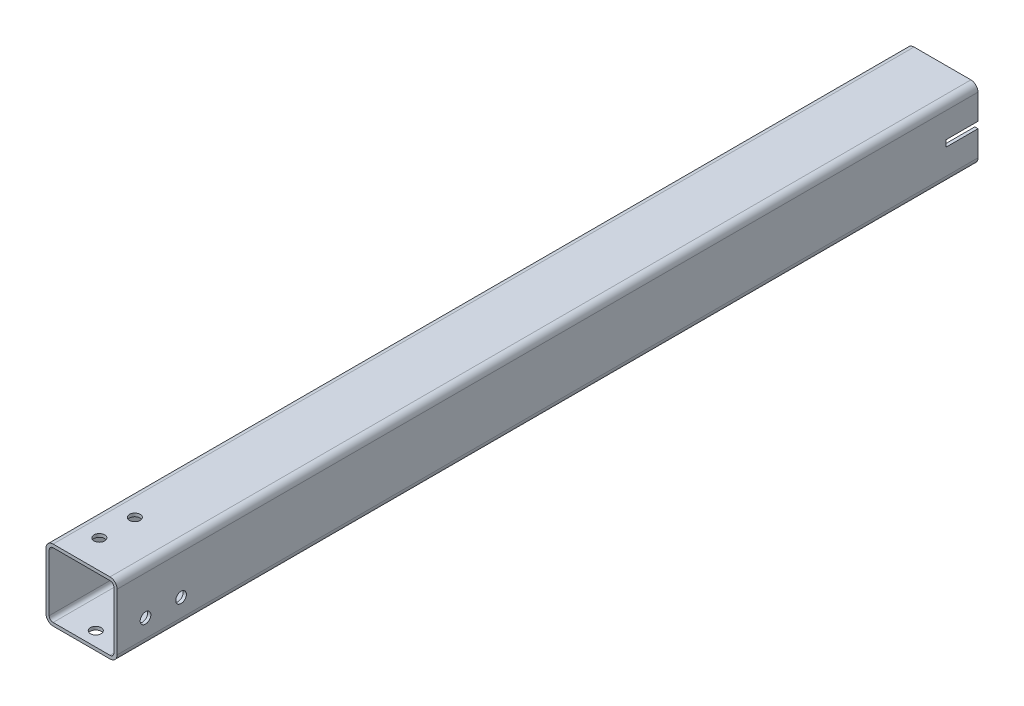
from build123d import *

# Parameters (mm, degrees)
BOSS_EXTRUDE1_DEPTH = 1211
CUT_EXTRUDE1_REACH  = 1218.15
SKETCH_1_R          = 7.5
CUT_EXTRUDE2_REACH  = 1218.15
SKETCH2_R           = 7.5
CUT_EXTRUDE3_REACH  = 1218.15
SKETCH3_R           = 7.5
SKETCH4_W           = 45
SKETCH4_H           = 9
CUT_EXTRUDE4_DEPTH  = 1217.150072976


with BuildPart() as part:
    # Sketch1 → Boss-Extrude1 (new body)
    with BuildSketch(Plane.XY):
        with BuildLine():
            Line((-40, -50), (40, -50))
            ThreePointArc((40, -50), (47.071067812, -47.071067812), (50, -40))
            Line((50, -40), (50, 40))
            ThreePointArc((50, 40), (47.071067812, 47.071067812), (40, 50))
            Line((40, 50), (-40, 50))
            ThreePointArc((-40, 50), (-47.071067812, 47.071067812), (-50, 40))
            Line((-50, 40), (-50, -40))
            ThreePointArc((-50, -40), (-47.071067812, -47.071067812), (-40, -50))
        make_face()
        with BuildLine():
            Line((-40, -45.5), (40, -45.5))
            ThreePointArc((40, -45.5), (43.889087297, -43.889087297), (45.5, -40))
            Line((45.5, -40), (45.5, 40))
            ThreePointArc((45.5, 40), (43.889087297, 43.889087297), (40, 45.5))
            Line((40, 45.5), (-40, 45.5))
            ThreePointArc((-40, 45.5), (-43.889087297, 43.889087297), (-45.5, 40))
            Line((-45.5, 40), (-45.5, -40))
            ThreePointArc((-45.5, -40), (-43.889087297, -43.889087297), (-40, -45.5))
        make_face(mode=Mode.SUBTRACT)
    extrude(amount=BOSS_EXTRUDE1_DEPTH)

    # 草图1 → Cut-Extrude1 (cut, up to next)
    with BuildSketch(Plane(origin=(50, 0, 0), x_dir=(0, 0, -1), z_dir=(1, 0, 0)), mode=Mode.PRIVATE) as cut_extrude1_sk1:
        with Locations((-1171, -15)):
            Circle(SKETCH_1_R)
    cut_extrude1_tool1 = extrude(cut_extrude1_sk1.sketch, amount=-CUT_EXTRUDE1_REACH, mode=Mode.PRIVATE) & part.part
    # 草图1 → Cut-Extrude1 (cut, up to next)
    with BuildSketch(Plane(origin=(50, 0, 0), x_dir=(0, 0, -1), z_dir=(1, 0, 0)), mode=Mode.PRIVATE) as cut_extrude1_sk2:
        with Locations((-1121, -15)):
            Circle(SKETCH_1_R)
    cut_extrude1_tool2 = extrude(cut_extrude1_sk2.sketch, amount=-CUT_EXTRUDE1_REACH, mode=Mode.PRIVATE) & part.part
    add(cut_extrude1_tool1.solids().sort_by_distance((50, -15, 1171))[0], mode=Mode.SUBTRACT)
    add(cut_extrude1_tool2.solids().sort_by_distance((50, -15, 1121))[0], mode=Mode.SUBTRACT)

    # Sketch2 → Cut-Extrude2 (cut, up to next)
    with BuildSketch(Plane.XZ.offset(50), mode=Mode.PRIVATE) as cut_extrude2_sk1:
        with Locations(Location((0, 1191, 0), (0, 0, 270))):
            Circle(SKETCH2_R)
    cut_extrude2_tool1 = extrude(cut_extrude2_sk1.sketch, amount=-CUT_EXTRUDE2_REACH, mode=Mode.PRIVATE) & part.part
    # Sketch2 → Cut-Extrude2 (cut, up to next)
    with BuildSketch(Plane.XZ.offset(50), mode=Mode.PRIVATE) as cut_extrude2_sk2:
        with Locations(Location((0, 1121, 0), (0, 0, 270))):
            Circle(SKETCH2_R)
    cut_extrude2_tool2 = extrude(cut_extrude2_sk2.sketch, amount=-CUT_EXTRUDE2_REACH, mode=Mode.PRIVATE) & part.part
    # Sketch2 → Cut-Extrude2 (cut, up to next)
    with BuildSketch(Plane.XZ.offset(50), mode=Mode.PRIVATE) as cut_extrude2_sk3:
        with Locations(Location((0, 20, 0), (0, 0, 270))):
            Circle(SKETCH2_R)
    cut_extrude2_tool3 = extrude(cut_extrude2_sk3.sketch, amount=-CUT_EXTRUDE2_REACH, mode=Mode.PRIVATE) & part.part
    add(cut_extrude2_tool1.solids().sort_by_distance((0, -50, 1191))[0], mode=Mode.SUBTRACT)
    add(cut_extrude2_tool2.solids().sort_by_distance((0, -50, 1121))[0], mode=Mode.SUBTRACT)
    add(cut_extrude2_tool3.solids().sort_by_distance((0, -50, 20))[0], mode=Mode.SUBTRACT)

    # Sketch3 → Cut-Extrude3 (cut, up to next)
    with BuildSketch(Plane(origin=(0, 50, 0), x_dir=(1, 0, 0), z_dir=(0, 1, 0)), mode=Mode.PRIVATE) as cut_extrude3_sk1:
        with Locations(Location((-15, -1171, 0), (0, 0, 270))):
            Circle(SKETCH3_R)
    cut_extrude3_tool1 = extrude(cut_extrude3_sk1.sketch, amount=-CUT_EXTRUDE3_REACH, mode=Mode.PRIVATE) & part.part
    # Sketch3 → Cut-Extrude3 (cut, up to next)
    with BuildSketch(Plane(origin=(0, 50, 0), x_dir=(1, 0, 0), z_dir=(0, 1, 0)), mode=Mode.PRIVATE) as cut_extrude3_sk2:
        with Locations(Location((-15, -1121, 0), (0, 0, 270))):
            Circle(SKETCH3_R)
    cut_extrude3_tool2 = extrude(cut_extrude3_sk2.sketch, amount=-CUT_EXTRUDE3_REACH, mode=Mode.PRIVATE) & part.part
    add(cut_extrude3_tool1.solids().sort_by_distance((-15, 50, 1171))[0], mode=Mode.SUBTRACT)
    add(cut_extrude3_tool2.solids().sort_by_distance((-15, 50, 1121))[0], mode=Mode.SUBTRACT)

    # Sketch4 → Cut-Extrude4 (cut, through all)
    with BuildSketch(Plane(origin=(50, 0, 0), x_dir=(0, 0, -1), z_dir=(1, 0, 0))):
        with Locations((-22.5, 0)):
            Rectangle(SKETCH4_W, SKETCH4_H)
    extrude(amount=-CUT_EXTRUDE4_DEPTH, mode=Mode.SUBTRACT)


solid = part.part
